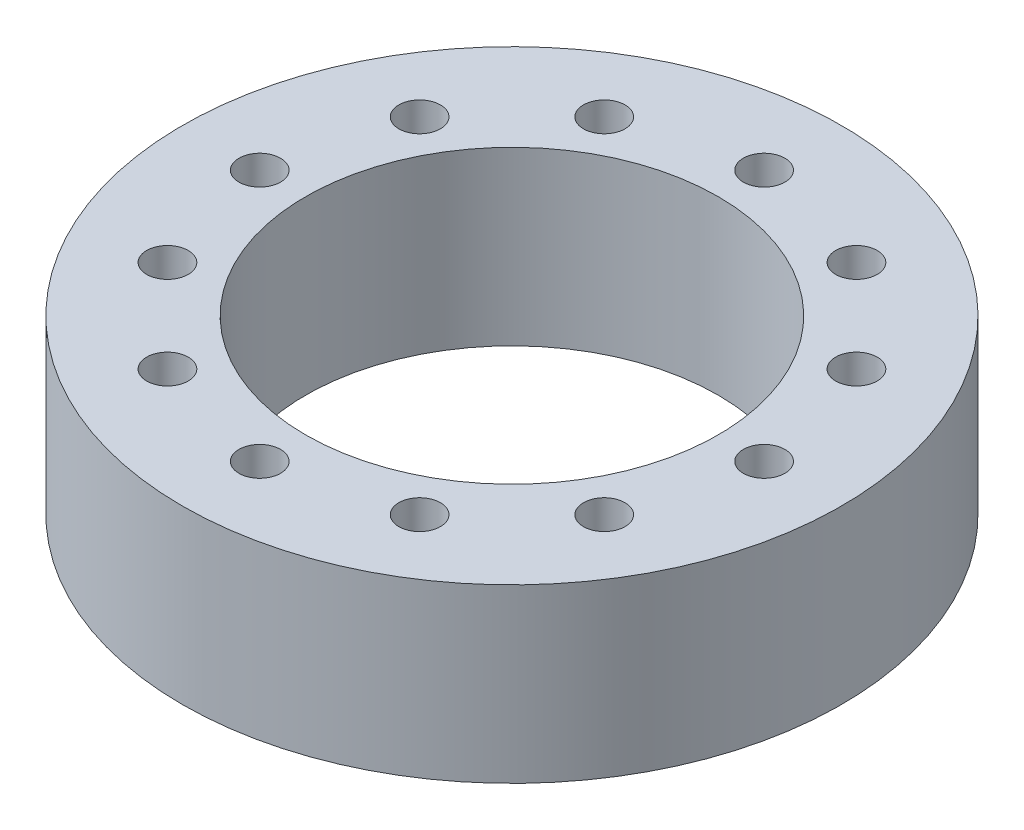
SolidWorks part; units mm, degrees
ref_plane "Front Plane" through (0, 0, 0) normal (0, 0, 1) x (1, 0, 0)
ref_plane "Top Plane" through (0, 0, 0) normal (0, 1, 0) x (1, 0, 0)
ref_plane "Right Plane" through (0, 0, 0) normal (1, 0, 0) x (0, 0, -1)
sketch "Sketch1" plane through (0, 0, 0) normal (0, 1, 0) x (1, 0, 0)
  circle A0 centre (0, 0) radius 115
  circle A1 centre (0, 0) radius 72
  circle A2 centre (0, 0) radius 88 construction
  circle A3 centre (0, 88) radius 7.25
  circle A4 centre (44, 76.2102) radius 7.25
  circle A5 centre (76.2102, 44) radius 7.25
  circle A6 centre (88, 0) radius 7.25
  circle A7 centre (76.2102, -44) radius 7.25
  circle A8 centre (44, -76.2102) radius 7.25
  circle A9 centre (0, -88) radius 7.25
  circle A10 centre (-44, -76.2102) radius 7.25
  circle A11 centre (-76.2102, -44) radius 7.25
  circle A12 centre (-88, 0) radius 7.25
  circle A13 centre (-76.2102, 44) radius 7.25
  circle A14 centre (-44, 76.2102) radius 7.25
  point P31 (0, 0)
  dimension "D1" = 230
  dimension "D2" = 144
  dimension "D3" = 176
  dimension "D4" = 14.5
extrude "Boss-Extrude1" add sketch "Sketch1" along normal blind 60
sketch "Sketch2" plane through (0, 0, 0) normal (0, -1, 0) x (1, 0, 0)
  circle A12 centre (0, 88) radius 11
  circle A13 centre (44, 76.2102) radius 11
  circle A14 centre (76.2102, 44) radius 11
  circle A15 centre (88, 0) radius 11
  circle A16 centre (76.2102, -44) radius 11
  circle A17 centre (44, -76.2102) radius 11
  circle A18 centre (0, -88) radius 11
  circle A19 centre (-44, -76.2102) radius 11
  circle A20 centre (-76.2102, -44) radius 11
  circle A21 centre (-88, 0) radius 11
  circle A22 centre (-76.2102, 44) radius 11
  circle A23 centre (-44, 76.2102) radius 11
  point P28 (0, 0)
  dimension "D1" = 22
extrude "Cut-Extrude1" cut sketch "Sketch2" against normal blind 30
